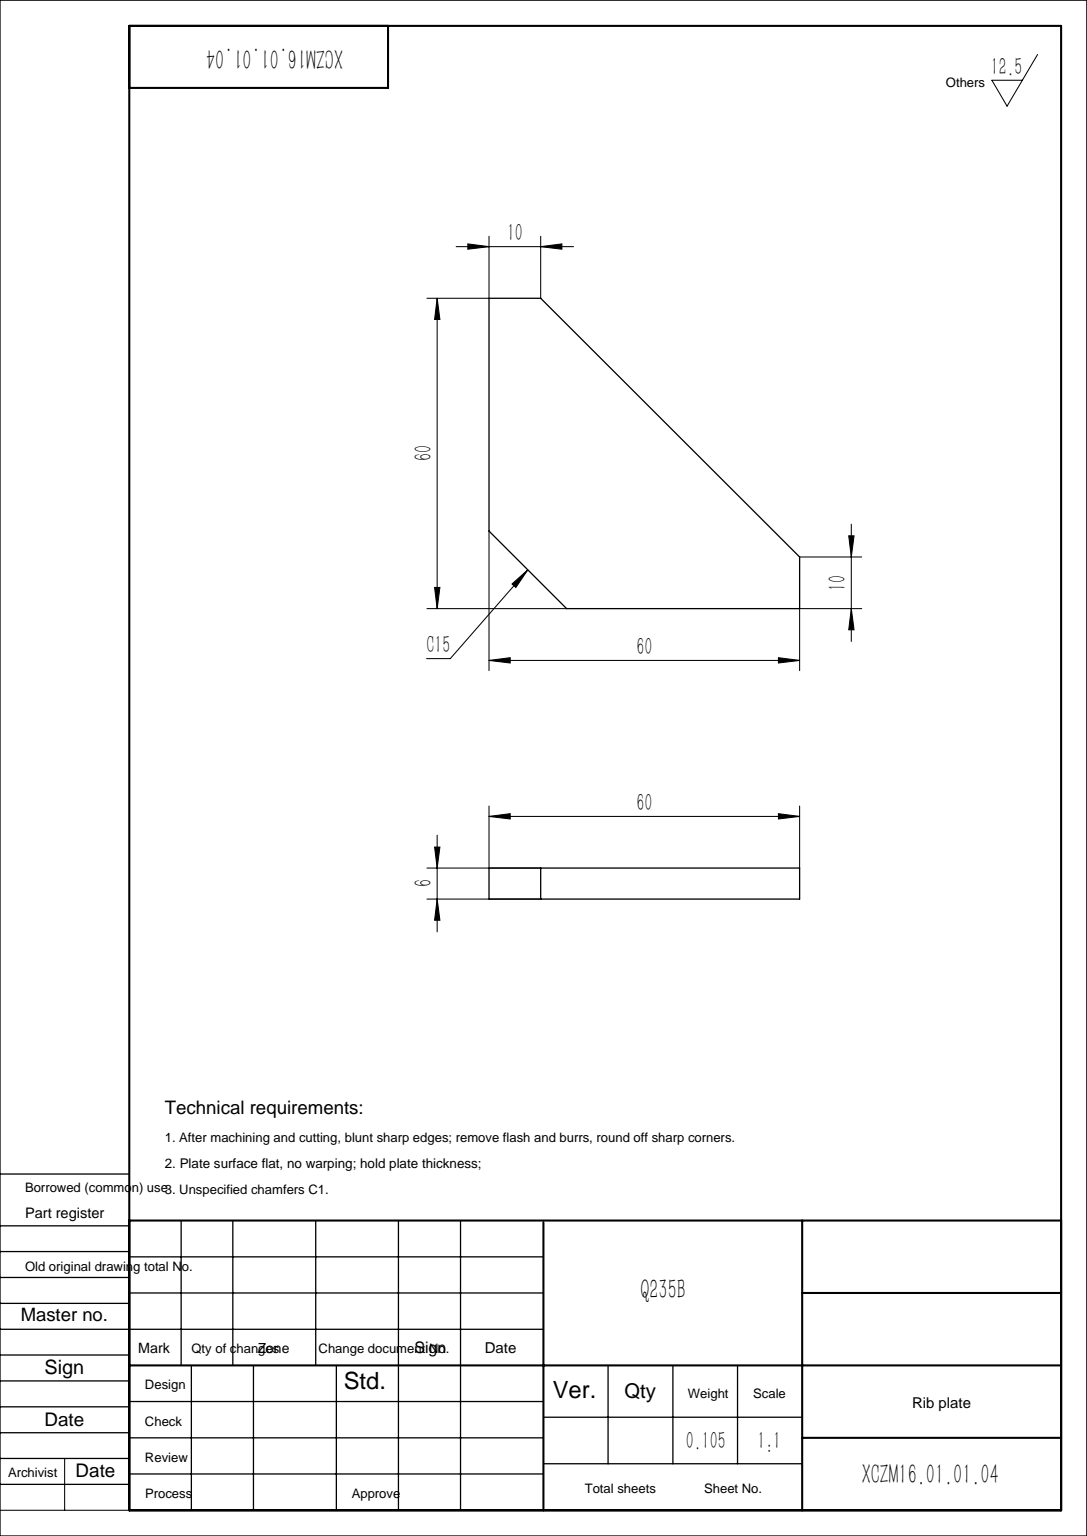
from build123d import *

# Parameters (mm, degrees)
BOSS_EXTRUDE1_DEPTH = 6
CHAMFER1_SIZE       = 15


with BuildPart() as part:
    # Sketch1 → Boss-Extrude1 (new body)
    with BuildSketch(Plane.XY):
        Polygon((0, 60), (0, 0), (60, 0), (60, 10), (10, 60), align=None)
    extrude(amount=BOSS_EXTRUDE1_DEPTH)

    # Chamfer1
    chamfer1_edges = [part.edges().sort_by_distance(p)[0] for p in [
        (0, 0, 3),
    ]]
    chamfer(chamfer1_edges, length=CHAMFER1_SIZE)


solid = part.part
